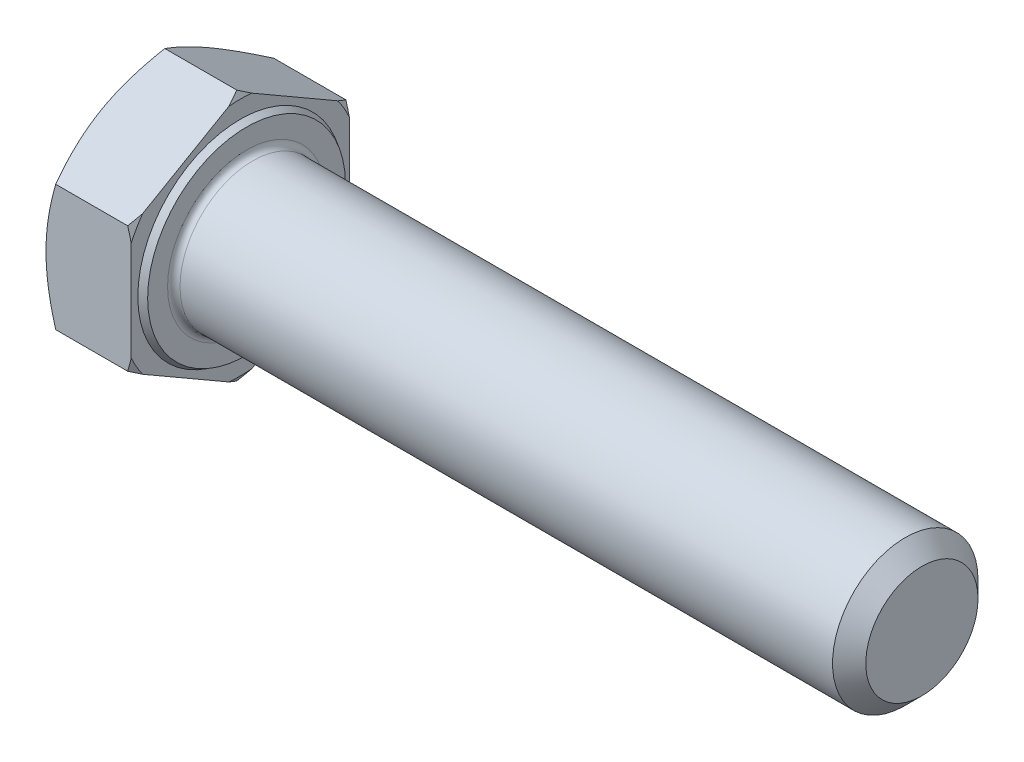
SolidWorks part; units mm, degrees
material "Q235B"
ref_plane "Front Plane" through (0, 0, 0) normal (0, 0, 1) x (1, 0, 0)
ref_plane "Top Plane" through (0, 0, 0) normal (0, 1, 0) x (1, 0, 0)
ref_plane "Right Plane" through (0, 0, 0) normal (1, 0, 0) x (0, 0, -1)
sketch "Dimension Sketch" plane through (0, 0, 0) normal (0, 0, 1) x (1, 0, 0)
  line L0 (0, 0) -> (34, 0) construction
  line L1 (0, 0) -> (0, 14) construction
  point P3 (2, 0)
  point P4 (0.6, 0)
  point P6 (0, 16.7)
  point P7 (0, 14.7)
  point P8 (0, 19.15)
  point P9 (22.78, 0)
  point P10 (8.8, 0)
  point P11 (5.85, 0)
  point P12 (0.6, 0)
  point P13 (21, 0)
  point P14 (65, 0)
  point P15 (31, 0)
  point P16 (55, 0)
  dimension "b(参考)" = 34
  dimension "P" = 2
  dimension "d" = 14
  dimension "c(max)" = 0.6
  dimension "da(max)" = 16.7
  dimension "ds(max)" = 14.7
  dimension "dw(min)" = 19.15
  dimension "e(min)" = 22.78
  dimension "k(公称)" = 8.8
  dimension "kw(min)" = 5.85
  dimension "r(min)" = 0.6
  dimension "s(公称)" = 21
  dimension "l" = 65
  dimension "lg(max)" = 31
  dimension "ls(min)" = 21
sketch "Sketch1" plane through (0, 0, 0) normal (1, 0, 0) x (0, 0, -1)
  line L0 (10.5, 6.0622) -> (10.5, -6.0622)
  line L1 (-10.5, 6.0622) -> (-10.5, -6.0622)
  line L2 (10.5, -6.0622) -> (0, -12.1244)
  line L3 (0, -12.1244) -> (-10.5, -6.0622)
  line L4 (10.5, 6.0622) -> (0, 12.1244)
  line L5 (0, 12.1244) -> (-10.5, 6.0622)
  point P6 (0, 10.6556)
  dimension "D1" = 22.78
  dimension "s" = 21
  dimension "D2" = 120
  dimension "D3" = 10.5
  dimension "D4" = 10.5
  dimension "D5" = 10.5
extrude "Boss-Extrude" add sketch "Sketch1" along normal blind 8.8
sketch "Sketch2" plane through (0, 0, 0) normal (0, 0, 1) x (1, 0, 0)
  line L0 (0, 6.0622) -> (0, -6.0622) construction
  line L1 (0, 0) -> (73.8, 0)
  line L2 (0, 0) -> (0, 7)
  line L3 (0, 7) -> (8.8, 7)
  line L4 (73.8, 0) -> (73.8, 5.268)
  line L5 (8.8, 12.1244) -> (8.8, 6.0622) construction
  line L7 (0, 0) -> (-51.1435, 0) construction
  line L8 (73.8, -5.268) -> (8.8, -7) construction
  line L9 (0, -7) -> (8.8, -7) construction
  line L10 (10.8, 7) -> (10.8, 0) construction
  line L11 (39.8, 7) -> (39.8, 0) construction
  line L12 (8.8, 6.0622) -> (8.8, -6.0622) construction
  line L13 (8.8, 7) -> (73.8, 7)
  line L14 (73.8, 7) -> (73.8, 5.268)
  dimension "l" = 65
  dimension "d" = 14
  dimension "Minor_dia" = 10.536
  dimension "p" = 2
  dimension "b" = 34
revolve "Boss-Revolve1" add sketch "Sketch2" angle 360 about L7
cosmetic thread "Cosmetic Thread1" parameters "D1"=34, "D2"=11.2
sketch "Sketch3" plane through (0, 0, 0) normal (0, 0, 1) x (1, 0, 0)
  line L0 (0, 10.5) -> (3.8246, 17.1244)
  line L1 (0, 12.1244) -> (0, 6.0622) construction
  line L2 (3.8246, 17.1244) -> (3.8246, 22.1244)
  line L3 (3.8246, 22.1244) -> (-10, 22.1244)
  line L4 (-10, 22.1244) -> (-10, 10.5)
  line L5 (-10, 10.5) -> (0, 10.5)
  line L6 (0, 0) -> (99.06, 0) construction
  line L7 (8.8, 12.1244) -> (0, 12.1244) construction
  dimension "D1" = 10.5
  dimension "D2" = 5
  dimension "D3" = 10
  dimension "D4" = 5
  dimension "Head_ch_ang" = 30
revolve "Cut-Revolve1" cut sketch "Sketch3" angle 360 about L6
sketch "Sketch5" plane through (0, 0, 0) normal (0, 0, 1) x (1, 0, 0)
  line L0 (8.8, 10.5) -> (4.9754, 17.1244)
  line L1 (8.8, 12.1244) -> (8.8, 6.0622) construction
  line L2 (4.9754, 17.1244) -> (4.9754, 22.1244)
  line L3 (4.9754, 22.1244) -> (14.9754, 22.1244)
  line L4 (14.9754, 22.1244) -> (14.9754, 10.5)
  line L5 (14.9754, 10.5) -> (8.8, 10.5)
  line L7 (8.8, 12.1244) -> (0.9378, 12.1244) construction
  line L8 (0, 0) -> (99.06, 0) construction
  line L9 (0, 0) -> (99.06, 0) construction
  dimension "D1" = 10.5
  dimension "D2" = 5
  dimension "D3" = 10
  dimension "Head_ch_ang" = 30
  dimension "D4" = 5
revolve "Cut-Revolve2" cut sketch "Sketch5" angle 360 about L8
sketch "Sketch4" plane through (0, 0, 0) normal (0, 0, 1) x (1, 0, 0)
  line L0 (8.7, 9.575) -> (8.7, 0) construction
  line L1 (8.8, 12.1244) -> (8.8, 6.0622) construction
  line L2 (8.8, 9.5173) -> (8.2, 9.8637)
  line L3 (8.8, 9.5173) -> (8.8, 22.1244)
  line L4 (8.8, 22.1244) -> (8.2, 22.1244)
  line L5 (0, 0) -> (95.25, 0) construction
  line L6 (-51.1435, 0) -> (0, 0) construction
  line L7 (8.2, 9.8637) -> (8.2, 22.1244)
  line L8 (7.8622, 12.1244) -> (0.9378, 12.1244) construction
  line L9 (8.8, 9.0933) -> (8.8, 10.5) construction
  line L10 (7.8622, 12.1244) -> (0.9378, 12.1244) construction
  point P15 (2.85, 12.1244)
  dimension "D1" = 120
  dimension "D2" = 10
  dimension "D3" = 0.1
  dimension "c" = 0.6
  dimension "D4" = 19.15
  dimension "D5" = 5.85
revolve "Cut-Revolve3" cut sketch "Sketch4" angle 360 about L5
chamfer "Chamfer" distance 1.6 angle 45 1 edges at (73.8, 0, -7)
sketch "Sketch9" plane through (0, 0, 0) normal (0, 0, 1) x (1, 0, 0)
  line L0 (8.8, -9.5173) -> (8.8, 9.5173) construction
  line L1 (72.2, 7) -> (8.8, 7) construction
  line L2 (0, 0) -> (8.8, 0) construction
  line L3 (8.8, 7.6) -> (8.8, 7)
  line L4 (8.8, 7) -> (9.4, 7)
  arc A0 (8.8, 7.6) -> (9.4, 7) centre (9.4, 7.6) ccw
  dimension "D1" = 0.6
revolve "Revolve1" add sketch "Sketch9" angle 360 about L2
sketch "Sketch6" plane through (0, 0, 0) normal (0, 0, 1) x (1, 0, 0)
  line L0 (71.2, -5.268) -> (70.2001, -7)
  line L1 (71.2, -5.268) -> (72.2, -7)
  line L2 (72.2, -7) -> (72.2, -12.1244)
  line L3 (-3.175, 0) -> (0, 0) construction
  line L4 (72.2, -7) -> (72.2, 7) construction
  line L5 (72.2, -12.1244) -> (70.2001, -12.1244)
  line L6 (70.2001, -12.1244) -> (70.2001, -7)
  line L7 (9.4, -7) -> (72.2, -7) construction
  line L9 (7.8622, -12.1244) -> (0.9378, -12.1244) construction
  dimension "Thread_minor" = 10.536
  dimension "SideAngle" = 60
  dimension "VeeAngle" = 60
revolve "Cut-Revolve4" [suppressed] cut sketch "Sketch6" angle 360 about L3
pattern_linear "LPattern1" [suppressed]
